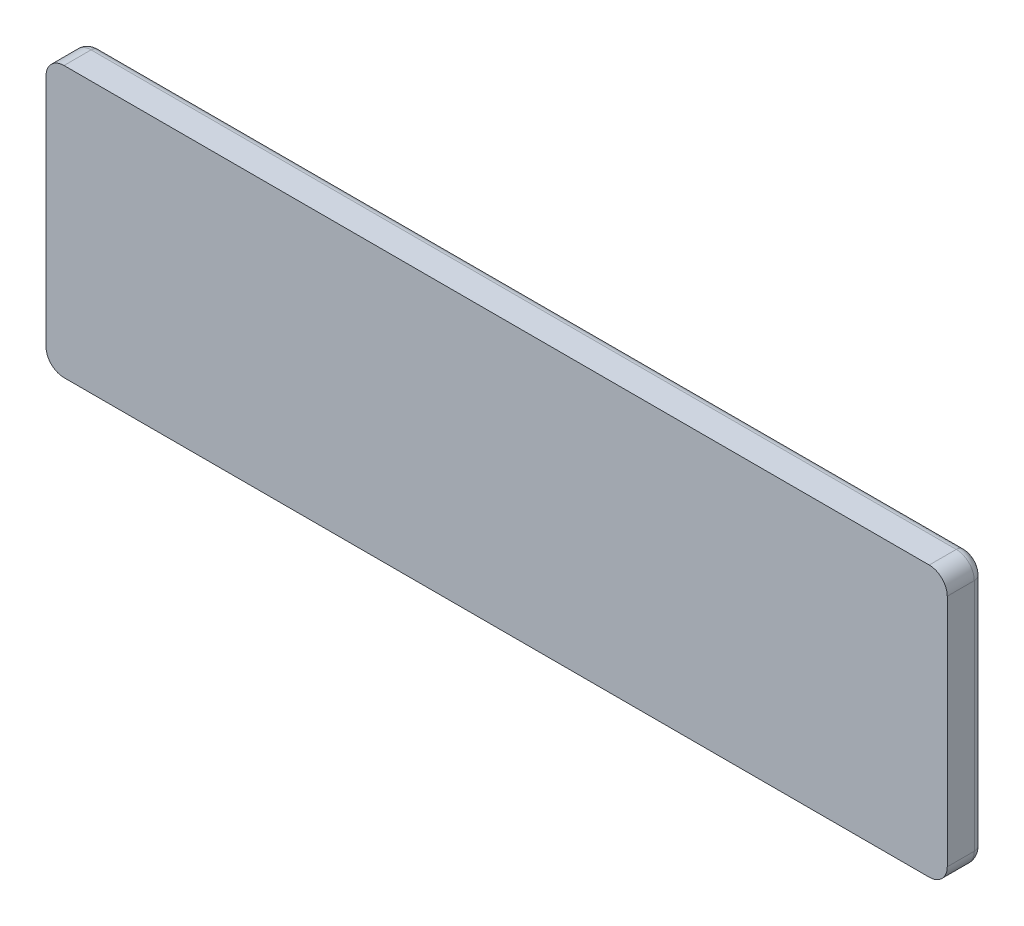
SolidWorks part; units mm, degrees
ref_plane "Front Plane" through (0, 0, 0) normal (0, 0, 1) x (1, 0, 0)
ref_plane "Top Plane" through (0, 0, 0) normal (0, 1, 0) x (1, 0, 0)
ref_plane "Right Plane" through (0, 0, 0) normal (1, 0, 0) x (0, 0, -1)
sketch "Sketch1" plane through (0, 0, 0) normal (0, 0, 1) x (1, 0, 0)
  line L0 (0, 150) -> (-50, 150)
  line L1 (0, 0) -> (450, 0)
  line L3 (0, 150) -> (450, 150)
  line L4 (450, 0) -> (450, 150)
  line L5 (-50, 150) -> (-50, 0)
  line L6 (-50, 0) -> (0, 0)
  dimension "D1" = 150
  dimension "D2" = 450
  dimension "D3" = 50
extrude "Boss-Extrude1" add sketch "Sketch1" along normal blind 20
sketch "Sketch2" plane through (0, 0, 0) normal (0, 0, -1) x (-1, 0, 0)
  line L0 (-450, 150) -> (50, 150) construction
  line L1 (-440, 140) -> (-425, 140)
  line L2 (-440, 140) -> (-440, 125)
  line L3 (-440, 125) -> (-425, 125)
  line L4 (-425, 140) -> (-425, 125)
  line L5 (-450, 0) -> (-450, 150) construction
  dimension "D1" = 15
  dimension "D2" = 15
  dimension "D3" = 10
  dimension "D4" = 10
extrude "Boss-Extrude2" add sketch "Sketch2" along normal blind 4
sketch "Sketch3" plane through (0, 0, 0) normal (0, 0, -1) x (-1, 0, 0)
  line L0 (-367.4537, 140) -> (-367.4537, 125)
  line L1 (-402.4537, 140) -> (-387.4537, 140)
  line L2 (-402.4537, 140) -> (-402.4537, 125)
  line L3 (-402.4537, 125) -> (-387.4537, 125)
  line L4 (-387.4537, 140) -> (-387.4537, 125)
  line L5 (-382.4537, 140) -> (-367.4537, 140)
  line L6 (-382.4537, 125) -> (-367.4537, 125)
  line L7 (-382.4537, 140) -> (-382.4537, 125)
  line L8 (-347.4537, 140) -> (-347.4537, 125)
  line L9 (-362.4537, 140) -> (-347.4537, 140)
  line L10 (-362.4537, 125) -> (-347.4537, 125)
  line L11 (-362.4537, 140) -> (-362.4537, 125)
  line L12 (-327.4537, 140) -> (-327.4537, 125)
  line L13 (-342.4537, 140) -> (-327.4537, 140)
  line L14 (-342.4537, 125) -> (-327.4537, 125)
  line L15 (-342.4537, 140) -> (-342.4537, 125)
  line L16 (-307.4537, 140) -> (-307.4537, 125)
  line L17 (-322.4537, 140) -> (-307.4537, 140)
  line L18 (-322.4537, 125) -> (-307.4537, 125)
  line L19 (-322.4537, 140) -> (-322.4537, 125)
  line L20 (-287.4537, 140) -> (-287.4537, 125)
  line L21 (-302.4537, 140) -> (-287.4537, 140)
  line L22 (-302.4537, 125) -> (-287.4537, 125)
  line L23 (-302.4537, 140) -> (-302.4537, 125)
  line L24 (-267.4537, 140) -> (-267.4537, 125)
  line L25 (-282.4537, 140) -> (-267.4537, 140)
  line L26 (-282.4537, 125) -> (-267.4537, 125)
  line L27 (-282.4537, 140) -> (-282.4537, 125)
  line L28 (-247.4537, 140) -> (-247.4537, 125)
  line L29 (-262.4537, 140) -> (-247.4537, 140)
  line L30 (-262.4537, 125) -> (-247.4537, 125)
  line L31 (-262.4537, 140) -> (-262.4537, 125)
  line L32 (-227.4537, 140) -> (-227.4537, 125)
  line L33 (-242.4537, 140) -> (-227.4537, 140)
  line L34 (-242.4537, 125) -> (-227.4537, 125)
  line L35 (-242.4537, 140) -> (-242.4537, 125)
  line L36 (-207.4537, 140) -> (-207.4537, 125)
  line L37 (-222.4537, 140) -> (-207.4537, 140)
  line L38 (-222.4537, 125) -> (-207.4537, 125)
  line L39 (-222.4537, 140) -> (-222.4537, 125)
  line L40 (-187.4537, 140) -> (-187.4537, 125)
  line L41 (-202.4537, 140) -> (-187.4537, 140)
  line L42 (-202.4537, 125) -> (-187.4537, 125)
  line L43 (-202.4537, 140) -> (-202.4537, 125)
  line L44 (-167.4537, 140) -> (-167.4537, 125)
  line L45 (-182.4537, 140) -> (-167.4537, 140)
  line L46 (-182.4537, 125) -> (-167.4537, 125)
  line L47 (-182.4537, 140) -> (-182.4537, 125)
  line L48 (-147.4537, 140) -> (-147.4537, 125)
  line L49 (-162.4537, 140) -> (-147.4537, 140)
  line L50 (-162.4537, 125) -> (-147.4537, 125)
  line L51 (-162.4537, 140) -> (-162.4537, 125)
  line L52 (-127.4537, 140) -> (-127.4537, 125)
  line L53 (-142.4537, 140) -> (-127.4537, 140)
  line L54 (-142.4537, 125) -> (-127.4537, 125)
  line L55 (-142.4537, 140) -> (-142.4537, 125)
  line L56 (-107.4537, 140) -> (-107.4537, 125)
  line L57 (-122.4537, 140) -> (-107.4537, 140)
  line L58 (-122.4537, 125) -> (-107.4537, 125)
  line L59 (-122.4537, 140) -> (-122.4537, 125)
  dimension "D1" = 15
  dimension "D2" = 15
extrude "Boss-Extrude3" add sketch "Sketch3" along normal blind 4
sketch "Sketch4" plane through (0, 0, 0) normal (0, 0, -1) x (-1, 0, 0)
  line L0 (-440, 125) -> (-425, 125) construction
  line L1 (-440, 115) -> (-425, 115)
  line L2 (-440, 115) -> (-440, 100)
  line L3 (-440, 100) -> (-425, 100)
  line L4 (-425, 115) -> (-425, 100)
  line L5 (-420, 115) -> (-420, 100)
  line L6 (-420, 115) -> (-405, 115)
  line L7 (-405, 115) -> (-405, 100)
  line L8 (-420, 100) -> (-405, 100)
  line L9 (-400, 115) -> (-400, 100)
  line L10 (-400, 115) -> (-385, 115)
  line L11 (-385, 115) -> (-385, 100)
  line L12 (-400, 100) -> (-385, 100)
  line L13 (-380, 115) -> (-380, 100)
  line L14 (-380, 115) -> (-365, 115)
  line L15 (-365, 115) -> (-365, 100)
  line L16 (-380, 100) -> (-365, 100)
  line L17 (-360, 115) -> (-360, 100)
  line L18 (-360, 115) -> (-345, 115)
  line L19 (-345, 115) -> (-345, 100)
  line L20 (-360, 100) -> (-345, 100)
  line L21 (-340, 115) -> (-340, 100)
  line L22 (-340, 115) -> (-325, 115)
  line L23 (-325, 115) -> (-325, 100)
  line L24 (-340, 100) -> (-325, 100)
  line L25 (-320, 115) -> (-320, 100)
  line L26 (-320, 115) -> (-305, 115)
  line L27 (-305, 115) -> (-305, 100)
  line L28 (-320, 100) -> (-305, 100)
  line L29 (-300, 115) -> (-300, 100)
  line L30 (-300, 115) -> (-285, 115)
  line L31 (-285, 115) -> (-285, 100)
  line L32 (-300, 100) -> (-285, 100)
  line L33 (-280, 115) -> (-280, 100)
  line L34 (-280, 115) -> (-265, 115)
  line L35 (-265, 115) -> (-265, 100)
  line L36 (-280, 100) -> (-265, 100)
  line L37 (-260, 115) -> (-260, 100)
  line L38 (-260, 115) -> (-245, 115)
  line L39 (-245, 115) -> (-245, 100)
  line L40 (-260, 100) -> (-245, 100)
  line L41 (-240, 115) -> (-240, 100)
  line L42 (-240, 115) -> (-225, 115)
  line L43 (-225, 115) -> (-225, 100)
  line L44 (-240, 100) -> (-225, 100)
  line L45 (-220, 115) -> (-220, 100)
  line L46 (-220, 115) -> (-205, 115)
  line L47 (-205, 115) -> (-205, 100)
  line L48 (-220, 100) -> (-205, 100)
  line L49 (-200, 115) -> (-200, 100)
  line L50 (-200, 115) -> (-185, 115)
  line L51 (-185, 115) -> (-185, 100)
  line L52 (-200, 100) -> (-185, 100)
  line L53 (-180, 115) -> (-180, 100)
  line L54 (-180, 115) -> (-165, 115)
  line L55 (-165, 115) -> (-165, 100)
  line L56 (-180, 100) -> (-165, 100)
  line L57 (-160, 115) -> (-160, 100)
  line L58 (-160, 115) -> (-145, 115)
  line L59 (-145, 115) -> (-145, 100)
  line L60 (-160, 100) -> (-145, 100)
  line L61 (-140, 115) -> (-140, 100)
  line L62 (-140, 115) -> (-120, 115)
  line L63 (-240, 27) -> (-225, 27)
  line L64 (-140, 100) -> (-120, 100)
  line L66 (-120, 115) -> (-105, 115)
  line L67 (-105, 115) -> (-105, 100)
  line L68 (-120, 100) -> (-105, 100)
  line L69 (-440, 93) -> (-440, 78)
  line L70 (-440, 93) -> (-425, 93)
  line L71 (-425, 93) -> (-425, 78)
  line L72 (-440, 78) -> (-425, 78)
  line L73 (-420, 93) -> (-420, 78)
  line L74 (-420, 93) -> (-405, 93)
  line L75 (-405, 93) -> (-405, 78)
  line L76 (-420, 78) -> (-405, 78)
  line L77 (-400, 93) -> (-400, 78)
  line L78 (-400, 93) -> (-385, 93)
  line L79 (-385, 93) -> (-385, 78)
  line L80 (-400, 78) -> (-385, 78)
  line L81 (-380, 93) -> (-380, 78)
  line L82 (-380, 93) -> (-365, 93)
  line L83 (-365, 93) -> (-365, 78)
  line L84 (-380, 78) -> (-365, 78)
  line L85 (-360, 93) -> (-360, 78)
  line L86 (-360, 93) -> (-345, 93)
  line L87 (-345, 93) -> (-345, 78)
  line L88 (-360, 78) -> (-345, 78)
  line L89 (-340, 93) -> (-340, 78)
  line L90 (-340, 93) -> (-325, 93)
  line L91 (-325, 93) -> (-325, 78)
  line L92 (-340, 78) -> (-325, 78)
  line L93 (-320, 93) -> (-320, 78)
  line L94 (-320, 93) -> (-305, 93)
  line L95 (-305, 93) -> (-305, 78)
  line L96 (-320, 78) -> (-305, 78)
  line L97 (-300, 93) -> (-300, 78)
  line L98 (-300, 93) -> (-285, 93)
  line L99 (-285, 93) -> (-285, 78)
  line L100 (-300, 78) -> (-285, 78)
  line L101 (-280, 93) -> (-280, 78)
  line L102 (-280, 93) -> (-265, 93)
  line L103 (-265, 93) -> (-265, 78)
  line L104 (-280, 78) -> (-265, 78)
  line L105 (-260, 93) -> (-260, 78)
  line L106 (-260, 93) -> (-245, 93)
  line L107 (-245, 93) -> (-245, 78)
  line L108 (-260, 78) -> (-245, 78)
  line L109 (-240, 93) -> (-240, 78)
  line L110 (-240, 93) -> (-225, 93)
  line L111 (-225, 93) -> (-225, 78)
  line L112 (-240, 78) -> (-225, 78)
  line L113 (-220, 93) -> (-220, 78)
  line L114 (-220, 93) -> (-205, 93)
  line L115 (-205, 93) -> (-205, 78)
  line L116 (-220, 78) -> (-205, 78)
  line L117 (-200, 93) -> (-200, 78)
  line L118 (-200, 93) -> (-185, 93)
  line L119 (-185, 93) -> (-185, 78)
  line L120 (-200, 78) -> (-185, 78)
  line L121 (-180, 93) -> (-180, 78)
  line L122 (-180, 93) -> (-165, 93)
  line L123 (-165, 93) -> (-165, 78)
  line L124 (-180, 78) -> (-165, 78)
  line L125 (-160, 93) -> (-160, 78)
  line L126 (-160, 93) -> (-145, 93)
  line L127 (-145, 93) -> (-145, 78)
  line L128 (-160, 78) -> (-145, 78)
  line L129 (-140, 93) -> (-140, 78)
  line L130 (-140, 93) -> (-120, 93)
  line L132 (-140, 78) -> (-120, 78)
  line L134 (-120, 93) -> (-105, 93)
  line L135 (-105, 93) -> (-105, 78)
  line L137 (-440, 71) -> (-440, 56)
  line L138 (-440, 71) -> (-425, 71)
  line L139 (-425, 71) -> (-425, 56)
  line L140 (-440, 56) -> (-425, 56)
  line L141 (-420, 71) -> (-420, 56)
  line L142 (-420, 71) -> (-405, 71)
  line L143 (-405, 71) -> (-405, 56)
  line L144 (-420, 56) -> (-405, 56)
  line L145 (-400, 71) -> (-400, 56)
  line L146 (-400, 71) -> (-385, 71)
  line L147 (-385, 71) -> (-385, 56)
  line L148 (-400, 56) -> (-385, 56)
  line L149 (-380, 71) -> (-380, 56)
  line L150 (-380, 71) -> (-365, 71)
  line L151 (-365, 71) -> (-365, 56)
  line L152 (-380, 56) -> (-365, 56)
  line L153 (-360, 71) -> (-360, 56)
  line L154 (-360, 71) -> (-345, 71)
  line L155 (-345, 71) -> (-345, 56)
  line L156 (-360, 56) -> (-345, 56)
  line L157 (-340, 71) -> (-340, 56)
  line L158 (-340, 71) -> (-325, 71)
  line L159 (-325, 71) -> (-325, 56)
  line L160 (-340, 56) -> (-325, 56)
  line L161 (-320, 71) -> (-320, 56)
  line L162 (-320, 71) -> (-305, 71)
  line L163 (-305, 71) -> (-305, 56)
  line L164 (-320, 56) -> (-305, 56)
  line L165 (-300, 71) -> (-300, 56)
  line L166 (-300, 71) -> (-285, 71)
  line L167 (-285, 71) -> (-285, 56)
  line L168 (-300, 56) -> (-285, 56)
  line L169 (-280, 71) -> (-280, 56)
  line L170 (-280, 71) -> (-265, 71)
  line L171 (-265, 71) -> (-265, 56)
  line L172 (-280, 56) -> (-265, 56)
  line L173 (-260, 71) -> (-260, 56)
  line L174 (-260, 71) -> (-245, 71)
  line L175 (-245, 71) -> (-245, 56)
  line L176 (-260, 56) -> (-245, 56)
  line L177 (-240, 71) -> (-240, 56)
  line L178 (-240, 71) -> (-225, 71)
  line L179 (-225, 71) -> (-225, 56)
  line L180 (-240, 56) -> (-225, 56)
  line L181 (-220, 71) -> (-220, 56)
  line L182 (-220, 71) -> (-205, 71)
  line L183 (-205, 71) -> (-205, 56)
  line L184 (-220, 56) -> (-205, 56)
  line L185 (-200, 71) -> (-200, 56)
  line L186 (-200, 71) -> (-185, 71)
  line L187 (-185, 71) -> (-185, 56)
  line L188 (-200, 56) -> (-185, 56)
  line L189 (-180, 71) -> (-180, 56)
  line L190 (-180, 71) -> (-165, 71)
  line L191 (-165, 71) -> (-165, 56)
  line L192 (-180, 56) -> (-165, 56)
  line L193 (-160, 71) -> (-160, 56)
  line L194 (-160, 71) -> (-145, 71)
  line L195 (-145, 71) -> (-145, 56)
  line L196 (-160, 56) -> (-145, 56)
  line L197 (-140, 71) -> (-140, 56)
  line L198 (-140, 71) -> (-125, 71)
  line L199 (-125, 71) -> (-125, 56)
  line L200 (-140, 56) -> (-125, 56)
  line L201 (-120, 78) -> (-120, 56)
  line L203 (-105, 78) -> (-105, 56)
  line L204 (-120, 56) -> (-105, 56)
  line L205 (-440, 49) -> (-440, 34)
  line L206 (-440, 49) -> (-425, 49)
  line L207 (-425, 49) -> (-425, 34)
  line L208 (-440, 34) -> (-425, 34)
  line L209 (-420, 49) -> (-420, 34)
  line L210 (-420, 49) -> (-405, 49)
  line L211 (-405, 49) -> (-405, 34)
  line L212 (-420, 34) -> (-405, 34)
  line L213 (-400, 49) -> (-400, 34)
  line L214 (-400, 49) -> (-385, 49)
  line L215 (-385, 49) -> (-385, 34)
  line L216 (-400, 34) -> (-385, 34)
  line L217 (-380, 49) -> (-380, 34)
  line L218 (-380, 49) -> (-365, 49)
  line L219 (-365, 49) -> (-365, 34)
  line L220 (-380, 34) -> (-365, 34)
  line L221 (-360, 49) -> (-360, 34)
  line L222 (-360, 49) -> (-345, 49)
  line L223 (-345, 49) -> (-345, 34)
  line L224 (-360, 34) -> (-345, 34)
  line L225 (-340, 49) -> (-340, 34)
  line L226 (-340, 49) -> (-325, 49)
  line L227 (-325, 49) -> (-325, 34)
  line L228 (-340, 34) -> (-325, 34)
  line L229 (-320, 49) -> (-320, 34)
  line L230 (-320, 49) -> (-305, 49)
  line L231 (-305, 49) -> (-305, 34)
  line L232 (-320, 34) -> (-305, 34)
  line L233 (-300, 49) -> (-300, 34)
  line L234 (-300, 49) -> (-285, 49)
  line L235 (-285, 49) -> (-285, 34)
  line L236 (-300, 34) -> (-285, 34)
  line L237 (-280, 49) -> (-280, 34)
  line L238 (-280, 49) -> (-265, 49)
  line L239 (-265, 49) -> (-265, 34)
  line L240 (-280, 34) -> (-265, 34)
  line L241 (-260, 49) -> (-260, 34)
  line L242 (-260, 49) -> (-245, 49)
  line L243 (-245, 49) -> (-245, 34)
  line L244 (-260, 34) -> (-245, 34)
  line L245 (-240, 49) -> (-240, 34)
  line L246 (-240, 49) -> (-225, 49)
  line L247 (-225, 49) -> (-225, 34)
  line L248 (-240, 34) -> (-225, 34)
  line L249 (-220, 49) -> (-220, 34)
  line L250 (-220, 49) -> (-205, 49)
  line L251 (-205, 49) -> (-205, 34)
  line L252 (-220, 34) -> (-205, 34)
  line L253 (-200, 49) -> (-200, 34)
  line L254 (-200, 49) -> (-185, 49)
  line L255 (-185, 49) -> (-185, 34)
  line L256 (-200, 34) -> (-185, 34)
  line L257 (-180, 49) -> (-180, 34)
  line L258 (-180, 49) -> (-165, 49)
  line L259 (-165, 49) -> (-165, 34)
  line L260 (-180, 34) -> (-165, 34)
  line L261 (-160, 49) -> (-160, 34)
  line L262 (-160, 49) -> (-145, 49)
  line L263 (-145, 49) -> (-145, 34)
  line L264 (-160, 34) -> (-145, 34)
  line L265 (-140, 49) -> (-140, 34)
  line L266 (-140, 49) -> (-125, 49)
  line L268 (-140, 34) -> (-125, 34)
  line L270 (-125, 49) -> (-105, 49)
  line L271 (-105, 49) -> (-105, 34)
  line L272 (-125, 34) -> (-105, 34)
  line L273 (-440, 27) -> (-440, 12)
  line L274 (-440, 27) -> (-425, 27)
  line L275 (-425, 27) -> (-425, 12)
  line L276 (-440, 12) -> (-425, 12)
  line L277 (-420, 27) -> (-420, 12)
  line L278 (-420, 27) -> (-405, 27)
  line L279 (-405, 27) -> (-405, 12)
  line L280 (-420, 12) -> (-405, 12)
  line L281 (-400, 27) -> (-400, 12)
  line L282 (-400, 27) -> (-385, 27)
  line L283 (-385, 27) -> (-385, 12)
  line L284 (-400, 12) -> (-385, 12)
  line L285 (-380, 27) -> (-380, 12)
  line L286 (-380, 27) -> (-365, 27)
  line L287 (-365, 27) -> (-365, 12)
  line L288 (-380, 12) -> (-365, 12)
  line L289 (-360, 27) -> (-360, 12)
  line L290 (-360, 27) -> (-345, 27)
  line L291 (-345, 27) -> (-345, 12)
  line L292 (-360, 12) -> (-345, 12)
  line L293 (-340, 27) -> (-340, 12)
  line L294 (-340, 27) -> (-320, 27)
  line L296 (-340, 12) -> (-325, 12)
  line L298 (-320, 27) -> (-300, 27)
  line L300 (-325, 12) -> (-305, 12)
  line L302 (-300, 27) -> (-280, 27)
  line L304 (-305, 12) -> (-280, 12)
  line L306 (-280, 27) -> (-260, 27)
  line L308 (-280, 12) -> (-260, 12)
  line L310 (-260, 27) -> (-240, 27)
  line L312 (-260, 12) -> (-240, 12)
  line L316 (-240, 12) -> (-220, 12)
  line L318 (-225, 27) -> (-205, 27)
  line L320 (-220, 12) -> (-200, 12)
  line L322 (-205, 27) -> (-185, 27)
  line L323 (-185, 27) -> (-185, 12)
  line L324 (-200, 12) -> (-185, 12)
  line L325 (-180, 27) -> (-180, 12)
  line L326 (-180, 27) -> (-165, 27)
  line L327 (-165, 27) -> (-165, 12)
  line L328 (-180, 12) -> (-165, 12)
  line L329 (-160, 27) -> (-160, 12)
  line L330 (-160, 27) -> (-145, 27)
  line L331 (-145, 27) -> (-145, 12)
  line L332 (-160, 12) -> (-145, 12)
  line L333 (-140, 27) -> (-140, 12)
  line L334 (-140, 27) -> (-125, 27)
  line L335 (-125, 27) -> (-125, 12)
  line L336 (-140, 12) -> (-125, 12)
  line L341 (-125, 115) -> (-125, 100) [skipped]
  line L342 (-120, 115) -> (-120, 100) [skipped]
  line L343 (-125, 93) -> (-125, 78) [skipped]
  line L344 (-120, 93) -> (-120, 78) [skipped]
  line L345 (-120, 78) -> (-105, 78) [skipped]
  line L346 (-120, 71) -> (-105, 71) [skipped]
  line L347 (-125, 49) -> (-125, 34) [skipped]
  line L348 (-120, 49) -> (-120, 34) [skipped]
  line L349 (-305, 27) -> (-305, 12) [skipped]
  line L350 (-300, 27) -> (-300, 12) [skipped]
  line L351 (-285, 27) -> (-285, 12) [skipped]
  line L352 (-280, 27) -> (-280, 12) [skipped]
  line L353 (-265, 27) -> (-265, 12) [skipped]
  line L354 (-260, 27) -> (-260, 12) [skipped]
  line L355 (-245, 27) -> (-245, 12) [skipped]
  line L356 (-240, 27) -> (-240, 12) [skipped]
  line L357 (-225, 27) -> (-225, 12) [skipped]
  line L358 (-220, 27) -> (-220, 12) [skipped]
  line L359 (-320, 27) -> (-320, 12) [skipped]
  line L360 (-325, 27) -> (-325, 12) [skipped]
  line L361 (-200, 27) -> (-200, 12) [skipped]
  line L362 (-205, 27) -> (-205, 12) [skipped]
  line L363 (-105, 27) -> (-105, 12) [skipped]
  line L364 (-120, 27) -> (-105, 27) [skipped]
  line L365 (-120, 27) -> (-120, 12) [skipped]
  line L366 (-120, 12) -> (-105, 12) [skipped]
  line L367 (-240, 27) -> (-205, 27) [skipped]
  dimension "D1" = 15
  dimension "D2" = 10
  dimension "D3" = 17
  dimension "D4" = 5
extrude "Boss-Extrude4" add sketch "Sketch4" along normal blind 4
sketch "Sketch5" plane through (0, 0, 0) normal (0, 0, -1) x (-1, 0, 0)
  line L0 (-107.4537, 125) -> (-107.4537, 140) construction
  line L1 (-97.4537, 140) -> (-82.4537, 140)
  line L2 (-97.4537, 140) -> (-97.4537, 125)
  line L3 (-97.4537, 125) -> (-82.4537, 125)
  line L4 (-82.4537, 140) -> (-82.4537, 125)
  line L5 (-62.4537, 140) -> (-62.4537, 125)
  line L6 (-77.4537, 140) -> (-62.4537, 140)
  line L7 (-77.4537, 125) -> (-62.4537, 125)
  line L8 (-77.4537, 140) -> (-77.4537, 125)
  line L9 (-42.4537, 140) -> (-42.4537, 125)
  line L10 (-57.4537, 140) -> (-42.4537, 140)
  line L11 (-57.4537, 125) -> (-42.4537, 125)
  line L12 (-57.4537, 140) -> (-57.4537, 125)
  line L13 (-77.4537, 115) -> (-77.4537, 100)
  line L14 (-97.4537, 115) -> (-82.4537, 115)
  line L15 (-97.4537, 115) -> (-97.4537, 100)
  line L16 (-97.4537, 100) -> (-82.4537, 100)
  line L17 (-82.4537, 115) -> (-82.4537, 100)
  line L18 (-77.4537, 115) -> (-62.4537, 115)
  line L19 (-62.4537, 115) -> (-62.4537, 100)
  line L20 (-77.4537, 100) -> (-62.4537, 100)
  line L21 (-57.4537, 115) -> (-57.4537, 100)
  line L22 (-57.4537, 115) -> (-42.4537, 115)
  line L23 (-42.4537, 115) -> (-42.4537, 100)
  line L24 (-57.4537, 100) -> (-42.4537, 100)
  line L25 (-97.4537, 93) -> (-97.4537, 78)
  line L26 (-97.4537, 93) -> (-82.4537, 93)
  line L27 (-82.4537, 93) -> (-82.4537, 78)
  line L28 (-97.4537, 78) -> (-82.4537, 78)
  line L29 (-77.4537, 93) -> (-77.4537, 78)
  line L30 (-77.4537, 93) -> (-62.4537, 93)
  line L31 (-62.4537, 93) -> (-62.4537, 78)
  line L32 (-77.4537, 78) -> (-62.4537, 78)
  line L33 (-57.4537, 93) -> (-57.4537, 78)
  line L34 (-57.4537, 93) -> (-42.4537, 93)
  line L35 (-42.4537, 93) -> (-42.4537, 78)
  line L36 (-57.4537, 78) -> (-42.4537, 78)
  line L38 (-77.4537, 49) -> (-62.4537, 49)
  line L39 (-77.4537, 49) -> (-77.4537, 34)
  line L40 (-77.4537, 34) -> (-62.4537, 34)
  line L41 (-62.4537, 49) -> (-62.4537, 34)
  line L42 (-97.4537, 27) -> (-82.4537, 27)
  line L43 (-97.4537, 27) -> (-97.4537, 12)
  line L44 (-97.4537, 12) -> (-82.4537, 12)
  line L45 (-82.4537, 27) -> (-82.4537, 12)
  line L46 (-77.4537, 27) -> (-62.4537, 27)
  line L47 (-77.4537, 27) -> (-77.4537, 12)
  line L48 (-77.4537, 12) -> (-62.4537, 12)
  line L49 (-62.4537, 27) -> (-62.4537, 12)
  line L50 (-57.4537, 27) -> (-42.4537, 27)
  line L51 (-57.4537, 27) -> (-57.4537, 12)
  line L52 (-57.4537, 12) -> (-42.4537, 12)
  line L53 (-42.4537, 27) -> (-42.4537, 12)
  dimension "D1" = 10
  dimension "D2" = 15
  dimension "D3" = 3
  dimension "D4" = 3
  dimension "D5" = 2
extrude "Boss-Extrude5" add sketch "Sketch5" along normal blind 4
sketch "Sketch6" plane through (0, 0, 0) normal (0, 0, -1) x (-1, 0, 0)
  line L0 (-10.4537, 115) -> (4.5463, 115)
  line L1 (-30.4537, 115) -> (-15.4537, 115)
  line L2 (-30.4537, 115) -> (-30.4537, 100)
  line L3 (-30.4537, 100) -> (-15.4537, 100)
  line L4 (-15.4537, 115) -> (-15.4537, 100)
  line L5 (4.5463, 115) -> (4.5463, 100)
  line L6 (-10.4537, 100) -> (4.5463, 100)
  line L7 (-10.4537, 115) -> (-10.4537, 100)
  line L8 (9.5463, 115) -> (24.5463, 115)
  line L9 (24.5463, 115) -> (24.5463, 100)
  line L10 (9.5463, 100) -> (24.5463, 100)
  line L11 (9.5463, 115) -> (9.5463, 100)
  line L12 (29.5463, 115) -> (44.5463, 115)
  line L13 (44.5463, 115) -> (44.5463, 100)
  line L14 (29.5463, 100) -> (44.5463, 100)
  line L15 (29.5463, 115) -> (29.5463, 100)
  line L16 (-30.4537, 93) -> (-15.4537, 93)
  line L17 (-15.4537, 93) -> (-15.4537, 78)
  line L18 (-30.4537, 78) -> (-15.4537, 78)
  line L19 (-30.4537, 93) -> (-30.4537, 78)
  line L20 (-10.4537, 93) -> (4.5463, 93)
  line L21 (4.5463, 93) -> (4.5463, 78)
  line L22 (-10.4537, 78) -> (4.5463, 78)
  line L23 (-10.4537, 93) -> (-10.4537, 78)
  line L24 (9.5463, 93) -> (24.5463, 93)
  line L25 (24.5463, 93) -> (24.5463, 78)
  line L26 (9.5463, 78) -> (24.5463, 78)
  line L27 (9.5463, 93) -> (9.5463, 78)
  line L28 (29.5463, 93) -> (44.5463, 93)
  line L29 (44.5463, 93) -> (44.5463, 78)
  line L31 (29.5463, 93) -> (29.5463, 78)
  line L32 (-30.4537, 71) -> (-15.4537, 71)
  line L33 (-15.4537, 71) -> (-15.4537, 56)
  line L34 (-30.4537, 56) -> (-15.4537, 56)
  line L35 (-30.4537, 71) -> (-30.4537, 56)
  line L36 (-10.4537, 71) -> (4.5463, 71)
  line L37 (4.5463, 71) -> (4.5463, 56)
  line L38 (-10.4537, 56) -> (4.5463, 56)
  line L39 (-10.4537, 71) -> (-10.4537, 56)
  line L40 (9.5463, 71) -> (24.5463, 71)
  line L41 (24.5463, 71) -> (24.5463, 56)
  line L42 (9.5463, 56) -> (24.5463, 56)
  line L43 (9.5463, 71) -> (9.5463, 56)
  line L45 (44.5463, 78) -> (44.5463, 56)
  line L46 (29.5463, 56) -> (44.5463, 56)
  line L47 (29.5463, 78) -> (29.5463, 56)
  line L48 (-30.4537, 49) -> (-15.4537, 49)
  line L49 (-15.4537, 49) -> (-15.4537, 34)
  line L50 (-30.4537, 34) -> (-15.4537, 34)
  line L51 (-30.4537, 49) -> (-30.4537, 34)
  line L52 (-10.4537, 49) -> (4.5463, 49)
  line L53 (4.5463, 49) -> (4.5463, 34)
  line L54 (-10.4537, 34) -> (4.5463, 34)
  line L55 (-10.4537, 49) -> (-10.4537, 34)
  line L56 (9.5463, 49) -> (24.5463, 49)
  line L57 (24.5463, 49) -> (24.5463, 34)
  line L58 (9.5463, 34) -> (24.5463, 34)
  line L59 (9.5463, 49) -> (9.5463, 34)
  line L60 (29.5463, 49) -> (44.5463, 49)
  line L61 (44.5463, 49) -> (44.5463, 27)
  line L63 (29.5463, 49) -> (29.5463, 27)
  line L64 (-30.4537, 27) -> (-15.4537, 27)
  line L66 (-30.4537, 12) -> (-10.4537, 12)
  line L67 (-30.4537, 27) -> (-30.4537, 12)
  line L68 (-15.4537, 27) -> (4.5463, 27)
  line L69 (4.5463, 27) -> (4.5463, 12)
  line L70 (-10.4537, 12) -> (4.5463, 12)
  line L72 (9.5463, 27) -> (24.5463, 27)
  line L73 (24.5463, 27) -> (24.5463, 12)
  line L74 (9.5463, 12) -> (24.5463, 12)
  line L75 (9.5463, 27) -> (9.5463, 12)
  line L77 (44.5463, 27) -> (44.5463, 12)
  line L78 (29.5463, 12) -> (44.5463, 12)
  line L79 (29.5463, 27) -> (29.5463, 12)
  line L80 (-42.4537, 100) -> (-42.4537, 115) construction
  line L81 (29.5463, 78) -> (44.5463, 78) [skipped]
  line L82 (29.5463, 71) -> (44.5463, 71) [skipped]
  line L83 (29.5463, 34) -> (44.5463, 34) [skipped]
  line L84 (29.5463, 27) -> (44.5463, 27) [skipped]
  line L85 (-10.4537, 27) -> (-10.4537, 12) [skipped]
  line L86 (-15.4537, 27) -> (-15.4537, 12) [skipped]
  dimension "D1" = 15
  dimension "D2" = 15
  dimension "D5" = 12
  dimension "D3" = 4
  dimension "D4" = 5
extrude "Boss-Extrude6" add sketch "Sketch6" along normal blind 4
sketch "Sketch7" plane through (0, 0, 0) normal (0, 0, -1) x (-1, 0, 0)
  line L0 (-42.4537, 125) -> (-42.4537, 140) construction
  circle A0 centre (-17.4537, 132.5) radius 2
  circle A1 centre (7.5463, 132.5) radius 2
  circle A2 centre (32.5463, 132.5) radius 2
  dimension "D1" = 4
  dimension "D3" = 25
  dimension "D2" = 3
extrude "Boss-Extrude7" add sketch "Sketch7" along normal blind 1
fillet "Fillet2" radius 10 4 edges at (-50, 150, 10) (-50, 0, 10) (450, 150, 10) (450, 0, 10)
fillet "Fillet3" radius 5 8 edges at (447.0711, 147.0711, 0) (450, 75, 0) (447.0711, 2.9289, 0) (200, 0, 0) (-47.0711, 2.9289, 0) (-50, 75, 0) (-47.0711, 147.0711, 0) (200, 150, 0)
